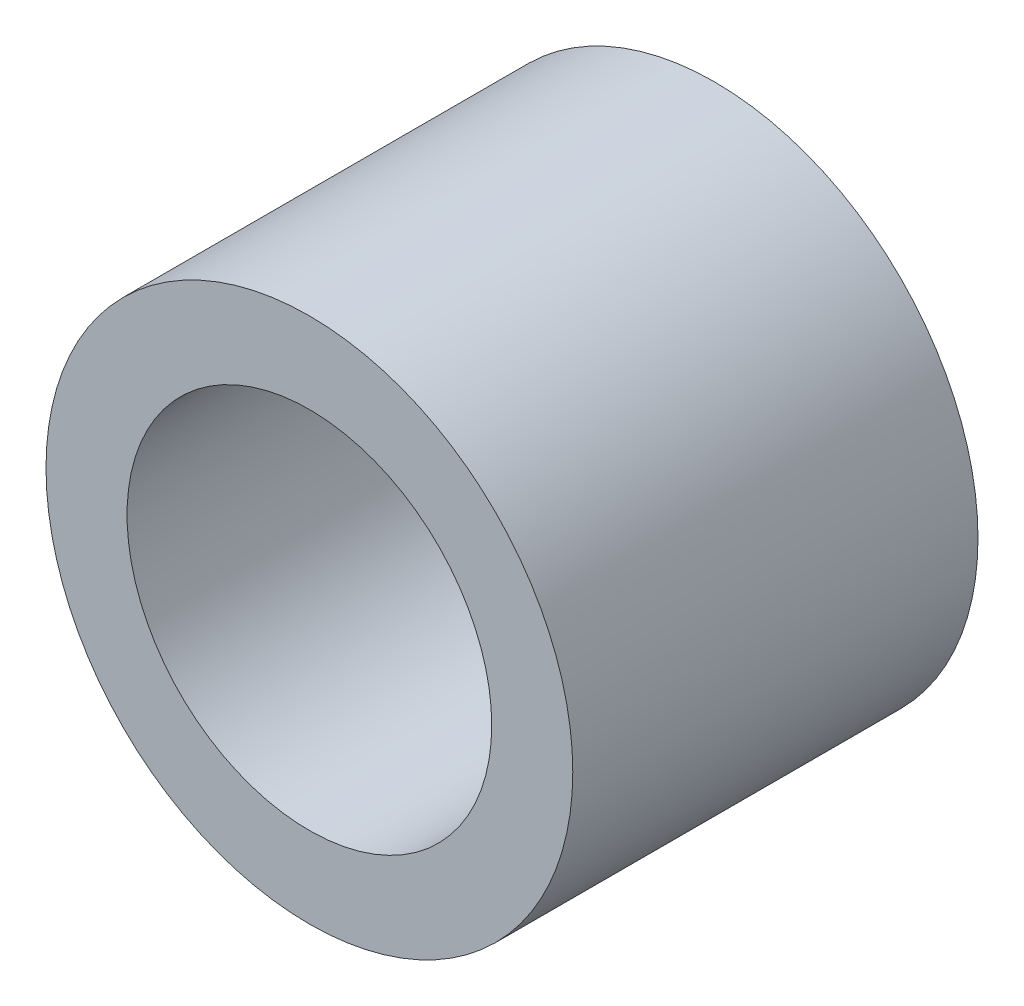
SolidWorks part; units mm, degrees
ref_plane "前视基准面" through (0, 0, 0) normal (0, 0, 1) x (1, 0, 0)
ref_plane "上视基准面" through (0, 0, 0) normal (0, 1, 0) x (1, 0, 0)
ref_plane "右视基准面" through (0, 0, 0) normal (1, 0, 0) x (0, 0, -1)
sketch "草图1" plane through (0, 0, 0) normal (0, 0, 1) x (1, 0, 0)
  circle A0 centre (0, 0) radius 32.5
  circle A1 centre (0, 0) radius 22.5
  dimension "D1" = 10
extrude "凸台-拉伸1" add sketch "草图1" along normal blind 50
